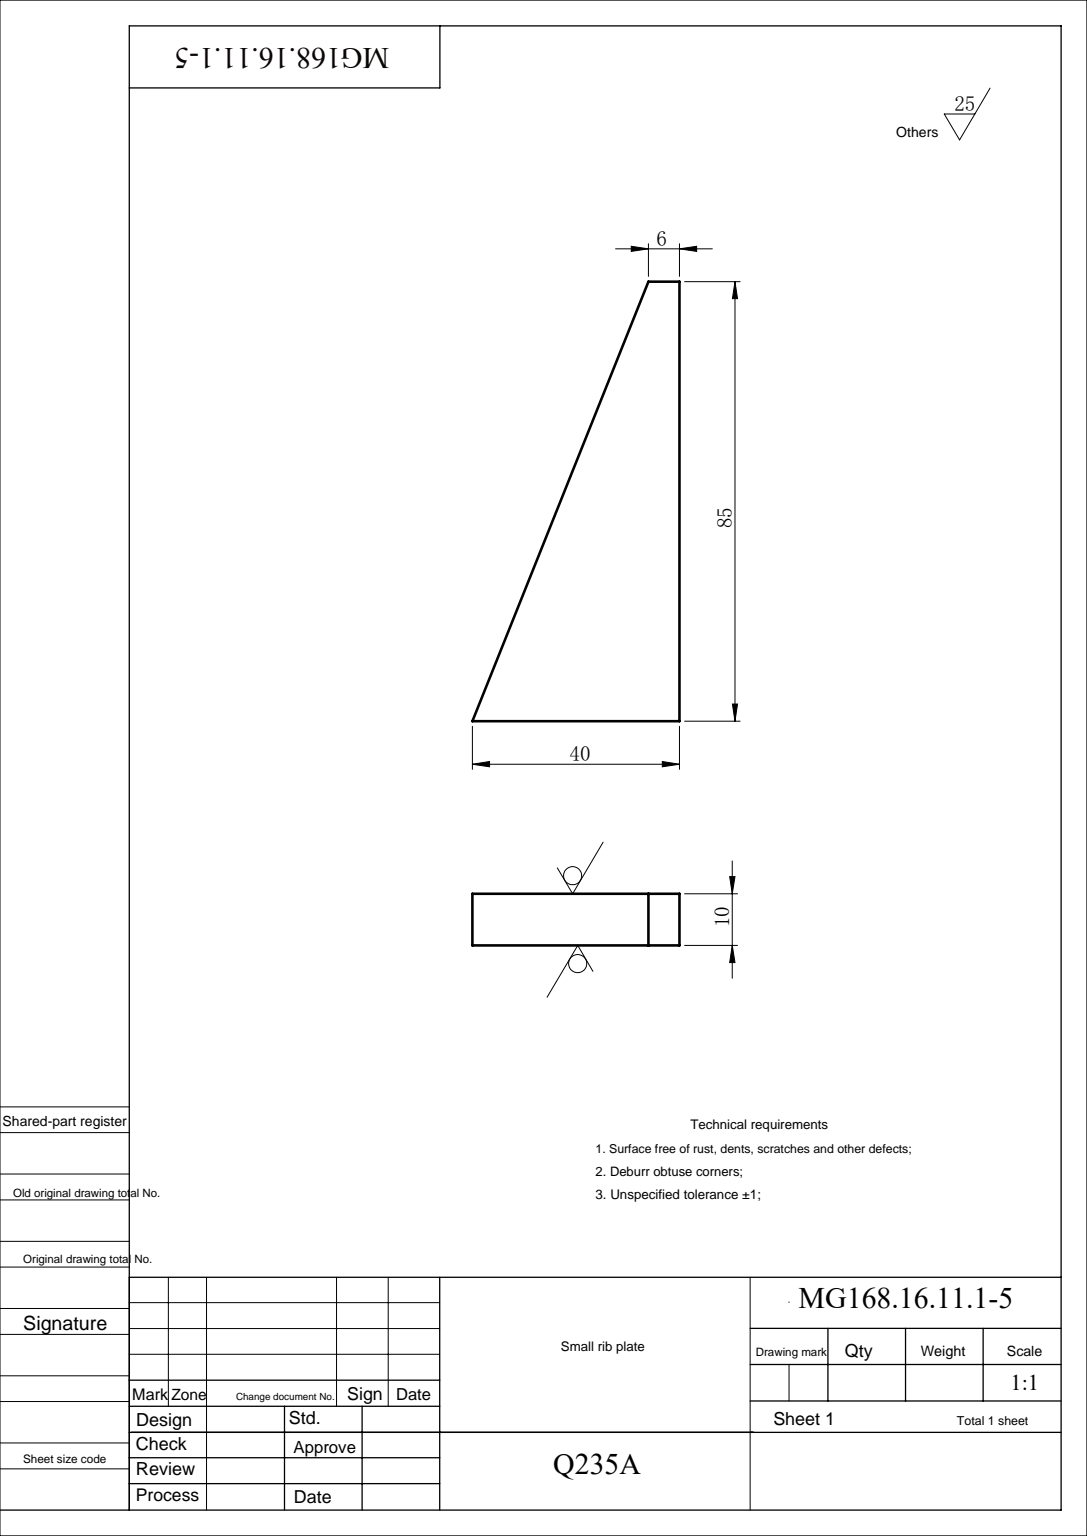
SolidWorks part; units mm, degrees
material "Q235A"
ref_plane "Front Plane" through (0, 0, 0) normal (0, 0, 1) x (1, 0, 0)
ref_plane "Top Plane" through (0, 0, 0) normal (0, 1, 0) x (1, 0, 0)
ref_plane "Right Plane" through (0, 0, 0) normal (1, 0, 0) x (0, 0, -1)
sketch "Sketch1" plane through (0, 0, 0) normal (0, 1, 0) x (1, 0, 0)
  line L0 (-6, 85) -> (-40, 0)
  line L1 (0, 0) -> (-40, 0)
  line L2 (0, 0) -> (0, 85)
  line L3 (0, 85) -> (-6, 85)
  dimension "D1" = 40
  dimension "D2" = 6
  dimension "D3" = 85
extrude "Boss-Extrude1" add sketch "Sketch1" along normal mid plane 10
